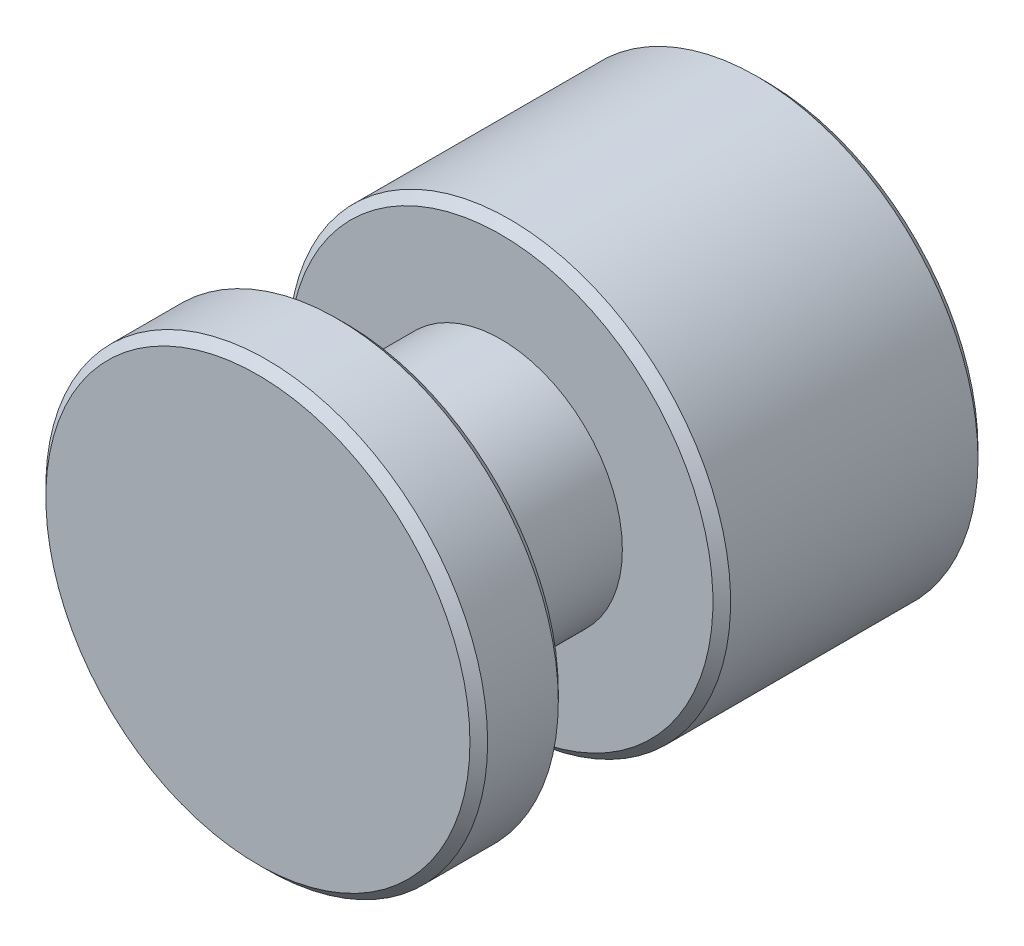
from build123d import *

# Parameters (mm, degrees)
SKETCH1_R             = 5
BOSS_EXTRUDE1_DEPTH   = 6
SKETCH2_R             = 2.75
BOSS_EXTRUDE2_DEPTH   = 3.5
SKETCH3_R             = 5
BOSS_EXTRUDE3_DEPTH   = 2
M4_TAPPED_HOLE1_D     = 3.3
M4_TAPPED_HOLE1_DEPTH = 8
M4_TAPPED_HOLE1_TIP   = 0.991420021
CHAMFER1_SIZE         = 0.2


with BuildPart() as part:
    # Sketch1 → Boss-Extrude1 (new body)
    with BuildSketch(Plane.XY):
        Circle(SKETCH1_R)
    extrude(amount=BOSS_EXTRUDE1_DEPTH)

    # Sketch2 → Boss-Extrude2 (add)
    with BuildSketch(Plane.XY.offset(6)):
        Circle(SKETCH2_R)
    extrude(amount=BOSS_EXTRUDE2_DEPTH)

    # Sketch3 → Boss-Extrude3 (add)
    with BuildSketch(Plane.XY.offset(9.5)):
        Circle(SKETCH3_R)
    extrude(amount=BOSS_EXTRUDE3_DEPTH)

    # M4 tapped hole1
    with Locations(Plane(origin=(0, 0, 0), x_dir=(-1, 0, 0), z_dir=(0, 0, -1))):
        with Locations((0, 0)):
            Hole(M4_TAPPED_HOLE1_D / 2, depth=M4_TAPPED_HOLE1_DEPTH)
            with Locations((0, 0, -(M4_TAPPED_HOLE1_DEPTH + M4_TAPPED_HOLE1_TIP / 2))):  # 118° drill point
                Cone(0, M4_TAPPED_HOLE1_D / 2, M4_TAPPED_HOLE1_TIP, mode=Mode.SUBTRACT)

    # Chamfer1
    chamfer1_edges = [part.edges().sort_by_distance(p)[0] for p in [
        (-5, 0, 0),
        (-5, 0, 6),
        (-5, 0, 9.5),
        (-5, 0, 11.5),
    ]]
    chamfer(chamfer1_edges, length=CHAMFER1_SIZE)


solid = part.part
